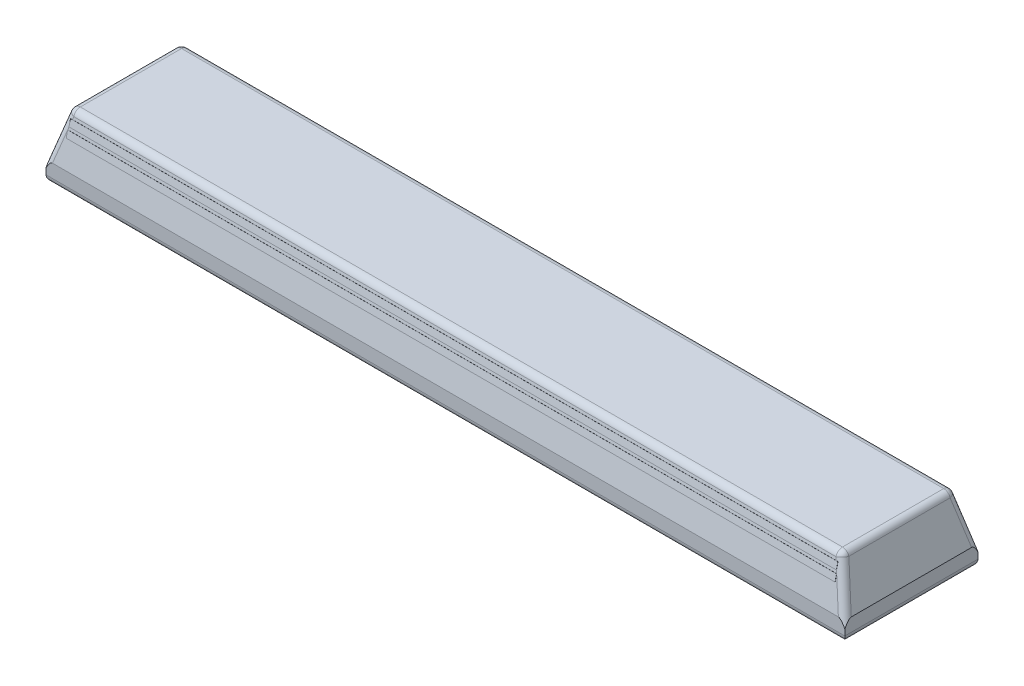
SolidWorks part; units mm, degrees
material "铸造碳钢"
ref_plane "Front Plane" through (0, 0, 0) normal (0, 0, 1) x (1, 0, 0)
ref_plane "Top Plane" through (0, 0, 0) normal (0, 1, 0) x (1, 0, 0)
ref_plane "Right Plane" through (0, 0, 0) normal (1, 0, 0) x (0, 0, -1)
sketch "Sketch1" plane through (0, 0, 0) normal (0, 0, 1) x (1, 0, 0)
  line L0 (100, 500) -> (5900, 500)
  line L1 (0, 150) -> (100, 500)
  line L2 (5900, 500) -> (6000, 150)
  line L3 (6000, 0) -> (0, 0)
  line L4 (6000, 150) -> (6000, 0)
  line L11 (0, 150) -> (0, 0)
extrude "Boss-Extrude1" add sketch "Sketch1" along normal mid plane 1000
sketch "Sketch2" plane through (0, 0, 500) normal (0, 0, 1) x (1, 0, 0)
  line L0 (3000, 500) -> (3000, 0) construction
  line L1 (5800, 300) -> (200, 300)
  line L2 (5800, 300) -> (5800, 200)
  line L3 (5800, 200) -> (200, 200)
  line L4 (200, 300) -> (200, 200)
  line L5 (5800, 300) -> (200, 200) construction
  line L6 (5800, 200) -> (200, 300) construction
  line L7 (5900, 500) -> (100, 500) construction
  line L8 (0, 0) -> (6000, 0) construction
  line L9 (6000, 0) -> (6000, 150) construction
  point P0 (3000, 250)
  dimension "D1" = 200
  dimension "D2" = 200
extrude "Cut-Extrude1" [suppressed] cut sketch "Sketch2" against normal through all
sketch "Sketch3" plane through (0, 0, 0) normal (-1, 0, 0) x (0, 0, 1)
  line L0 (0, 500) -> (0, 0) construction
  line L1 (500, 500) -> (-500, 500) construction
  line L2 (500, 0) -> (-500, 0) construction
  circle A0 centre (0, 750) radius 145
  dimension "D1" = 290
  dimension "D2" = 750
extrude "Cut-Extrude2" [suppressed] cut sketch "Sketch3" against normal through all both and the other way through all
sketch "Sketch4" plane through (0, 0, 0) normal (0, -1, 0) x (-1, 0, 0)
  line L0 (-3000, -500) -> (-3000, 500) construction
  line L1 (0, -500) -> (-6000, -500) construction
  line L2 (0, 500) -> (-6000, 500) construction
  line L4 (-500, -250) -> (-5500, -250) construction
  line L5 (-500, -250) -> (-500, 250) construction
  line L6 (-500, 250) -> (-5500, 250) construction
  line L7 (-5500, -250) -> (-5500, 250) construction
  line L8 (-500, -250) -> (-5500, 250) construction
  line L9 (-500, 250) -> (-5500, -250) construction
  line L10 (-6000, -500) -> (-6000, 500) construction
  circle A0 centre (-500, -250) radius 100
  circle A1 centre (-500, 250) radius 100
  circle A2 centre (-5500, 250) radius 100
  circle A3 centre (-5500, -250) radius 100
  circle A4 centre (-3000, -250) radius 100
  circle A5 centre (-3000, 250) radius 100
  point P6 (-3000, 0)
  dimension "D3" = 200
  dimension "D1" = 500
  dimension "D2" = 250
extrude "Boss-Extrude2" add sketch "Sketch4" along normal blind 100
sketch "Sketch5" plane through (6000, 0, 0) normal (1, 0, 0) x (0, 0, -1)
  line L0 (-420, 500) -> (-500, 150)
  line L1 (-500, 500) -> (500, 500) construction
  line L2 (-500, 150) -> (-500, 500)
  line L3 (-500, 150) -> (-500, 500) construction
  line L4 (-500, 500) -> (-420, 500)
  line L5 (500, 500) -> (500, 150)
  line L6 (500, 150) -> (420, 500)
  line L7 (420, 500) -> (500, 500)
  dimension "D1" = 80
extrude "Cut-Extrude3" cut sketch "Sketch5" against normal through all both and the other way through all
fillet "Fillet1" radius 50 12 edges at (5900, 500, 0) (100, 500, 0) (6000, 0, 0) (3000, 0, -500) (3000, 0, 500) (0, 0, 0) (50, 325, 460) (50, 325, -460) (3000, 500, -420) (3000, 500, 420)
fillet "Fillet2" radius 20 6 edges at (500, -100, -350) (5500, -100, 150) (5500, -100, -350) (3000, -100, -350) (3000, -100, 150) (500, -100, 150)
sketch "Sketch8" plane through (0, 116.059, 507.758) normal (0, 0.2228, 0.9749) x (1, 0, 0)
  line L0 (3000, 353.9819) -> (3000, 34.8164) construction
  line L1 (5862.2849, 353.9819) -> (137.7151, 353.9819) construction
  line L2 (48.8176, 34.8164) -> (5951.1824, 34.8164) construction
  line L3 (5951.1824, 34.8164) -> (5862.2849, 353.9819) construction
  line L4 (118.2179, 333.9819) -> (5881.7821, 333.9819)
  line L5 (118.2179, 333.9819) -> (118.2179, 283.9819)
  line L6 (118.2179, 283.9819) -> (5881.7821, 283.9819)
  line L7 (5881.7821, 333.9819) -> (5881.7821, 283.9819)
  line L8 (118.2179, 333.9819) -> (5881.7821, 283.9819) construction
  line L9 (118.2179, 283.9819) -> (5881.7821, 333.9819) construction
  line L11 (112.6473, 213.9819) -> (5887.3527, 213.9819)
  line L12 (112.6473, 213.9819) -> (112.6473, 263.9819)
  line L13 (112.6473, 263.9819) -> (5887.3527, 263.9819)
  line L14 (5887.3527, 213.9819) -> (5887.3527, 263.9819)
  line L15 (112.6473, 213.9819) -> (5887.3527, 263.9819) construction
  line L16 (112.6473, 263.9819) -> (5887.3527, 213.9819) construction
  point P6 (3000, 308.9819)
  point P13 (3000, 238.9819)
  dimension "D1" = 50
  dimension "D2" = 20
  dimension "D3" = 20
extrude "Boss-Extrude3" add sketch "Sketch8" along normal blind 1
equation "\"D4@Sketch1\"=\"D2@Sketch1\""
equation "\"D6@Sketch1\"=\"D5@Sketch1\""
